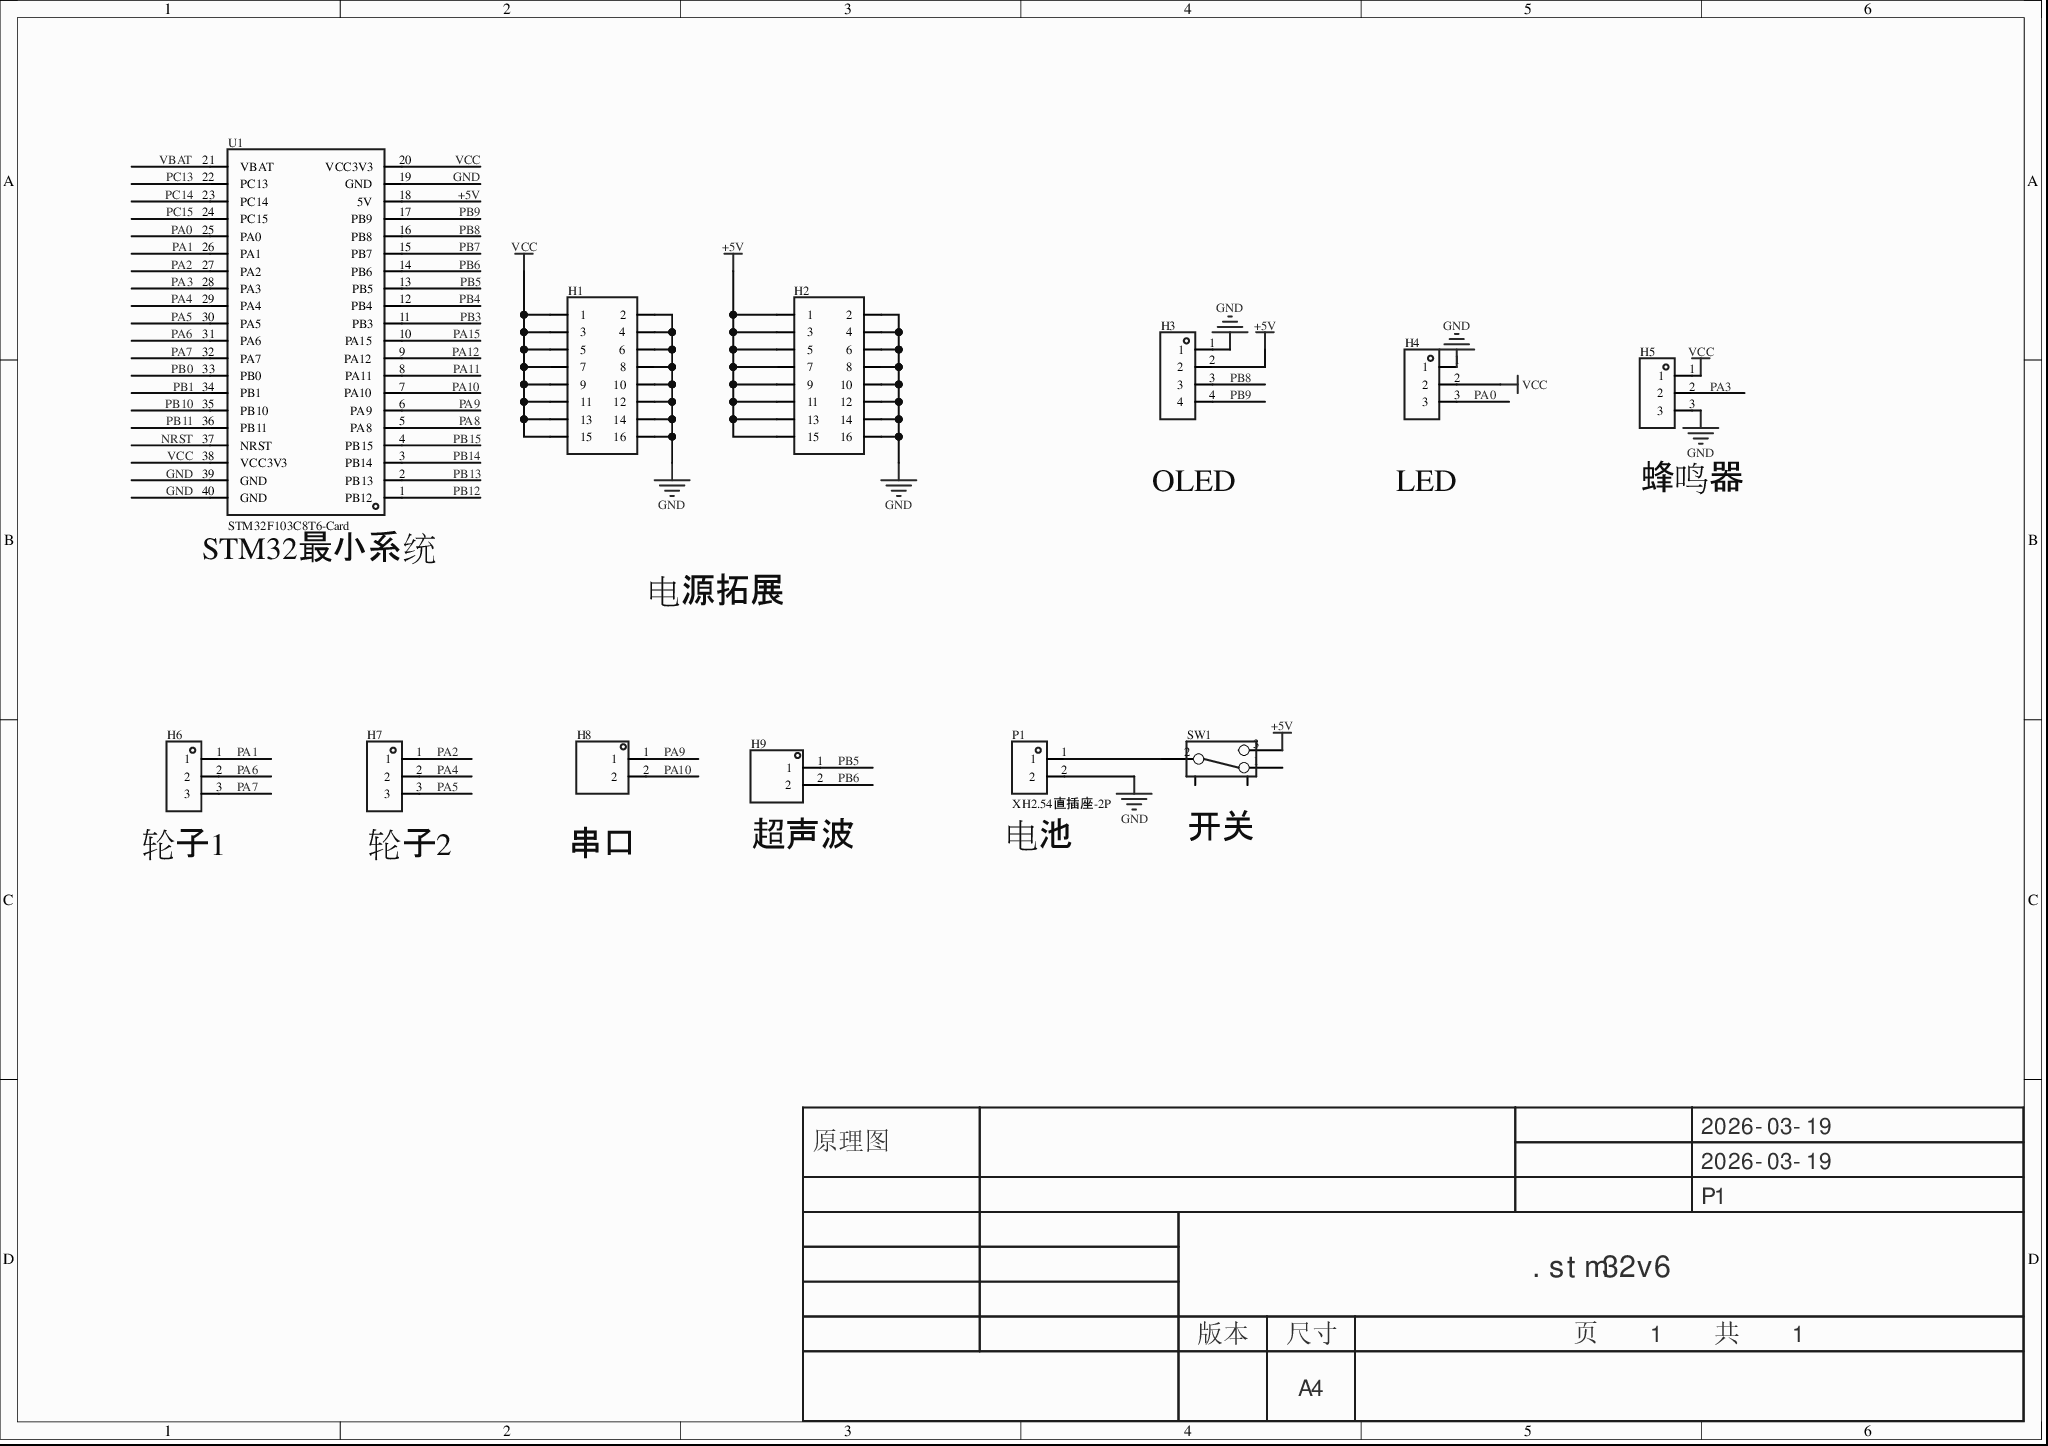
[diagram p0: MISC51854-3.schdoc]
# Altium project MISC51854-2.PrjPcb
1 sheet, 12 parts. Net scope: global (net labels, ports and power ports of the same name join across sheets).
Board file: MISC51854.pcbdoc

## Sheet MISC51854-3.schdoc
size 297 x 209 mm; Version: V1.0; @Project Name: MISC51854; @Page Count: 1; @Update Date: 2026-03-19; @Create Date: 2026-03-19; @Schematic Name: MISC51854; @Page No: 1; @Create Time: 23:22:16; @Update Time: 17:32:40; @Board Name: MISC51854

### Parts
H1  (no value)  [HDR-TH_16P-P2.54-V-F-R2-C8-S2.54-1]
H2  (no value)  [HDR-TH_16P-P2.54-V-F-R2-C8-S2.54-1]
H3  (no value)  [HDR-TH_4P-P2.54-V-F]
H4  (no value)  [HDR-TH_3P-P2.54-V-F]
H5  (no value)  [HDR-TH_3P-P2.54-V-F]
H6  (no value)  [HDR-TH_3P-P2.54-V-F]
H7  (no value)  [HDR-TH_3P-P2.54-V-F]
H8  (no value)  [HDR-TH_2P-P2.54-V-M-1]
H9  (no value)  [HDR-TH_2P-P2.54-V-M-1]
P1  XH2.54直插座-2P  [CONN-TH_XH2.54-2P]
SW1  (no value)  [拨动开关_侧]
U1  STM32F103C8T6-Card  [CONN-TH_L53.3-W22.9_STM32F103C8T6-CARD]

### Nets
+5V: H2.1 H2.3 H2.5 H2.7 H2.9 H2.11 H2.13 H2.15 H3.2 SW1.3 U1.18(5V)
GND: H1.2 H1.4 H1.6 H1.8 H1.10 H1.12 H1.14 H1.16 H2.2 H2.4 H2.6 H2.8 H2.10 H2.12 H2.14 H2.16 H3.1 H4.1 H5.3 P1.2 U1.19(GND) U1.39(GND) U1.40(GND)
VCC: H1.1 H1.3 H1.5 H1.7 H1.9 H1.11 H1.13 H1.15 H4.2 H5.1 U1.20(VCC3V3) U1.38(VCC3V3)
NRST: U1.37(NRST)
PA0: H4.3 U1.25(PA0)
PA1: H6.1 U1.26(PA1)
PA2: H7.1 U1.27(PA2)
PA3: H5.2 U1.28(PA3)
PA4: H7.2 U1.29(PA4)
PA5: H7.3 U1.30(PA5)
PA6: H6.2 U1.31(PA6)
PA7: H6.3 U1.32(PA7)
PA8: U1.5(PA8)
PA9: H8.1 U1.6(PA9)
PA10: H8.2 U1.7(PA10)
PA11: U1.8(PA11)
PA12: U1.9(PA12)
PA15: U1.10(PA15)
PB0: U1.33(PB0)
PB1: U1.34(PB1)
PB3: U1.11(PB3)
PB4: U1.12(PB4)
PB5: H9.1 U1.13(PB5)
PB6: H9.2 U1.14(PB6)
PB7: U1.15(PB7)
PB8: H3.3 U1.16(PB8)
PB9: H3.4 U1.17(PB9)
PB10: U1.35(PB10)
PB11: U1.36(PB11)
PB12: U1.1(PB12)
PB13: U1.2(PB13)
PB14: U1.3(PB14)
PB15: U1.4(PB15)
PC13: U1.22(PC13)
PC14: U1.23(PC14)
PC15: U1.24(PC15)
VBAT: U1.21(VBAT)
NetP1_1: P1.1 SW1.2

Not connected (* = marked no-connect by the designer): SW1 1 4 5

### Notes on the sheet
- (near H3) OLED
- (near H4) LED
- (near H5) 蜂鸣器
- (near U1) STM32最小系统
- 电源拓展
- (near H6) 轮子1
- (near H7) 轮子2
- (near H8) 串口
- (near H9) 超声波
- (near P1) 电池
- (near SW1) 开关
- Labels drawn without touching a wire or pin: VCC
- 2026-03-19
- 原理图
- P1
- .stm32v6
- 版本
- 尺寸
- A4
- 页    1    共    1

### Library data of the parts
H1 H2 = HDR-F_2.54_2x8: Symbol: HDR-F-2.54_2x8; ConvertToPcb: yes; ModelId: f6b5f7d40ec74b809fbaeebc5002f6e00819f05c4eef4c71ace90d822a990e87; ModelName: HDR2.54-F-LI-2X8P; ModelTransform: 799.99844,200,0,0,0,0,0,0,-118.11; Device: HDR-F_2.54_2x8; AddInBom: yes; SupplierPart: C30734; Supplier Footprint: 插件; FootprintName: HDR-TH_16P-P2.54-V-F-R2-C8-S2.54-1
H3 = HDR-F_2.54_1x4P: Symbol: 2.54-1*4P母; ConvertToPcb: yes; ModelId: d187812051054f85879fcaa51a310d8e0819f05c4eef4c71ace90d822a990e87; ModelTransform: 419.6842,98.464,0,0,0,0,0,0,-118.11; Device: HDR-F_2.54_1x4P; AddInBom: yes; SupplierPart: C2718488; Supplier Footprint: 插件; FootprintName: HDR-TH_4P-P2.54-V-F; ModelName: HDR-TH_4P-P2.54-V-F
H4-H7 = HDR-F_2.54_1x3P: Symbol: PM254V-11-03-H85; ConvertToPcb: yes; ModelId: f3b3cc5aae9641bf9e56fc160cef875b; ModelName: HDR2.54-F-LI-1X3P; ModelTransform: 299.9994,100,0,0,0,0,0,0,-118.11; Device: HDR-F_2.54_1x3P; AddInBom: yes; SupplierPart: C541850; Supplier Footprint: 插件; FootprintName: HDR-TH_3P-P2.54-V-F
H8 H9 = HDR-M_2.54_1x2P: Symbol: 210S-1*2P L=11.6MMGold-plated black; ConvertToPcb: yes; ModelId: 79b2e9f2d70a4d68a1b7098f27c6d4c50819f05c4eef4c71ace90d822a990e87; ModelName: HDR-M-2.54_1x2; ModelTransform: 200,100,0,0,0,0,0,0,-118.11; Device: HDR-M_2.54_1x2P; AddInBom: yes; SupplierPart: C124375; Supplier Footprint: 插件; FootprintName: HDR-TH_2P-P2.54-V-M-1
P1 = XH2.54直插座-2P: AddInBom: yes; ModelId: c3cc11bd8b8748c1ae6bc231aac3a1ff0819f05c4eef4c71ace90d822a990e87; ModelTransform: 296.889,230.315,0,0,0,0,0,26.653,-137.795; Symbol: XH2.54直插座-2P; Device: XH2.54直插座-2P; LCSC Part Name: XH2.54直插座-2P; SupplierPart: C9900016957; ManufacturerPart: XH2.54直插座-2P; Supplier Footprint: XH2.54-2; JLCPCB Part Class: Extended Part; Supplier: LCSC; ConvertToPcb: yes; FootprintName: CONN-TH_XH2.54-2P; ModelName: CONN-TH_XH2.54-2P
SW1 = 拨动开关_侧: Symbol: 拨动开关; ConvertToPcb: yes; ModelId: 10ea2cc5ba004a75b38812aadef1031f0819f05c4eef4c71ace90d822a990e87; ModelName: SW-TH_SK-12D07-VG3; ModelTransform: 337.98,287.46,295.24,0,0,0,0,-57,-110; Device: 拨动开关_侧; AddInBom: yes; Supplier Footprint: 插件; FootprintName: 拨动开关_侧
U1 = STM32F103C8T6-Card: AddInBom: yes; Symbol: STM32F103C8T6-CARD; Device: STM32F103C8T6-Card; LCSC Part Name: STM32F103C8T6-Card; SupplierPart: C9900077949; ManufacturerPart: STM32F103C8T6-Card; Supplier Footprint: 插件; Supplier: LCSC; ConvertToPcb: yes; FootprintName: CONN-TH_L53.3-W22.9_STM32F103C8T6-CARD